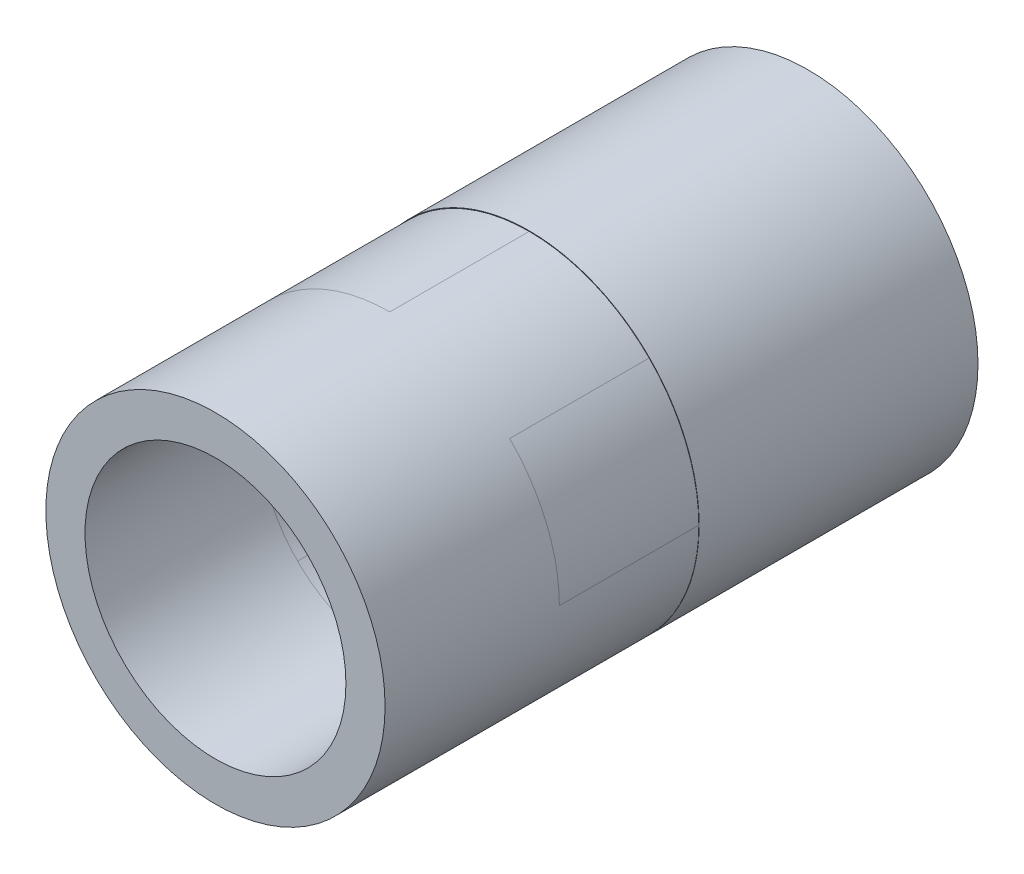
SolidWorks part; units mm, degrees
ref_plane "Front Plane" through (0, 0, 0) normal (0, 0, 1) x (1, 0, 0)
ref_plane "Top Plane" through (0, 0, 0) normal (0, 1, 0) x (1, 0, 0)
ref_plane "Right Plane" through (0, 0, 0) normal (1, 0, 0) x (0, 0, -1)
other "Configuration Table"
sketch "Sketch1" plane through (0, 0, 0) normal (0, 0, 1) x (1, 0, 0)
  circle A1 centre (0, 0.0078) radius 3.75
  circle A2 centre (0, 0.0078) radius 4.8729
extrude "Boss-Extrude1" add sketch "Sketch1" along normal blind 4 and the other way blind 4
sketch "Sketch3" plane through (0, 0, 4) normal (0, 0, 1) x (1, 0, 0)
  line L0 (0, 3.7578) -> (0, 4.8651)
  line L1 (-2.6555, 2.6555) -> (-3.4401, 3.4401)
  line L2 (3.7578, 0) -> (4.8651, 0)
  line L3 (2.6555, 2.6555) -> (3.4401, 3.4401)
  line L4 (0, -3.7578) -> (0, -4.8651)
  line L5 (2.6555, -2.6555) -> (3.4401, -3.4401)
  line L6 (-3.7578, 0) -> (-4.8651, 0)
  line L7 (-2.6555, -2.6555) -> (-3.4401, -3.4401)
  arc A0 (0, 4.8651) -> (-3.4401, 3.4401) centre (0, 0) ccw
  circle A2 centre (0, 0.0078) radius 3.75 construction
  arc A3 (0, 3.7578) -> (-2.6555, 2.6555) centre (0, 0.0078) ccw
  arc A4 (4.8651, 0) -> (3.4401, 3.4401) centre (0, 0) ccw
  arc A5 (3.7578, 0) -> (2.6555, 2.6555) centre (0.0078, 0) ccw
  arc A6 (0, -4.8651) -> (3.4401, -3.4401) centre (0, 0) ccw
  arc A7 (0, -3.7578) -> (2.6555, -2.6555) centre (0, -0.0078) ccw
  arc A8 (-4.8651, 0) -> (-3.4401, -3.4401) centre (0, 0) ccw
  arc A9 (-3.7578, 0) -> (-2.6555, -2.6555) centre (-0.0078, 0) ccw
  point P25 (0, 0)
  dimension "D1" = 45
  dimension "D2" = 4
extrude "Boss-Extrude2" add sketch "Sketch3" along normal blind 4
sketch "Sketch4" plane through (0, 0, 8) normal (0, 0, 1) x (1, 0, 0)
  circle A0 centre (0, 0) radius 4.8651
  circle A1 centre (0, 0) radius 3.7422
extrude "Boss-Extrude3" add sketch "Sketch4" along normal blind 5 separate body
sketch "Sketch5" plane through (0, 0, 8) normal (0, 0, -1) x (-1, 0, 0)
  line L0 (3.7578, 0) -> (4.8651, 0)
  line L1 (3.4401, 3.4401) -> (2.6555, 2.6555)
  line L2 (0, -3.7578) -> (0, -4.8651)
  line L3 (3.4401, -3.4401) -> (2.6555, -2.6555)
  line L4 (0, 3.7578) -> (0, 4.8651) construction
  line L5 (0, 3.7578) -> (0, 4.8651)
  line L6 (-3.4401, 3.4401) -> (-2.6555, 2.6555) construction
  line L7 (-3.4401, 3.4401) -> (-2.6555, 2.6555)
  line L8 (-3.7578, 0) -> (-4.8651, 0)
  line L9 (-3.4401, -3.4401) -> (-2.6555, -2.6555)
  arc A0 (0, 3.7578) -> (-2.6572, 2.6572) centre (0, 0) ccw
  arc A1 (3.7578, 0) -> (2.6572, 2.6572) centre (0, 0) ccw
  arc A2 (4.8651, 0) -> (3.4401, 3.4401) centre (0, 0) ccw
  arc A3 (0, -3.7578) -> (2.6572, -2.6572) centre (0, 0) ccw
  arc A4 (0, -4.8651) -> (3.4401, -3.4401) centre (0, 0) ccw
  arc A5 (-3.7578, 0) -> (-2.6572, -2.6572) centre (0, 0) ccw
  circle A7 centre (0, 0) radius 4.8651
  arc A8 (0, 4.8651) -> (-3.4401, 3.4401) centre (0, 0) ccw
  arc A10 (-4.8651, 0) -> (-3.4401, -3.4401) centre (0, 0) ccw
  point P25 (0, 0)
  circle M3 centre (0, 0) radius 4.8651
  dimension "D2" = 4
  dimension "D1" = 0
extrude "Boss-Extrude4" add sketch "Sketch5" along normal blind 4 contours A0 L5 L7 M3 | A1 L0 L1 M3 | A5 L8 L9 M3 | A3 L2 L3 M3
